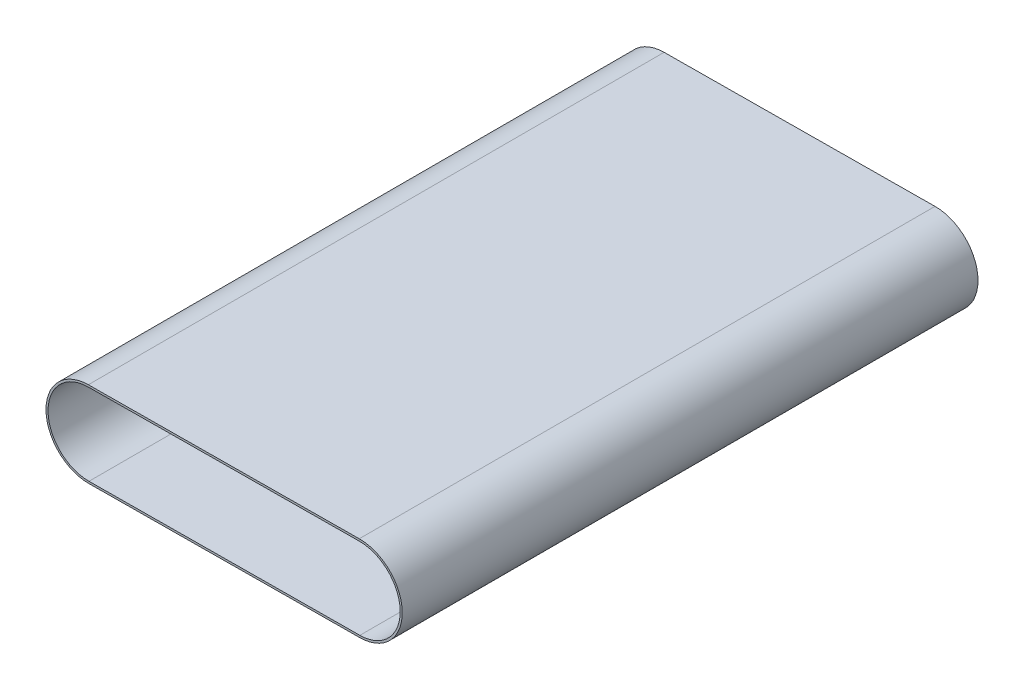
from build123d import *

# Parameters (mm, degrees)
EXTRUDE_1_DEPTH = 850


with BuildPart() as part:
    # 草图1 → 凸台-拉伸1 (new body)
    with BuildSketch(Plane.XY.offset(425)):
        with BuildLine():
            Line((662.463520786, 1437.017242521), (1062.402598848, 1440.036279946))
            ThreePointArc((1062.402598848, 1440.036279946), (1125.876361221, 1377.513632127), (1063.353713402, 1314.039869754))
            Line((1063.353713402, 1314.039869754), (663.414635339, 1311.020832329))
            ThreePointArc((663.414635339, 1311.020832329), (599.940872967, 1373.543480148), (662.463520786, 1437.017242521))
        make_face()
        with BuildLine():
            Line((662.48616637, 1434.017327992), (1062.425244433, 1437.036365417))
            ThreePointArc((1062.425244433, 1437.036365417), (1122.876446692, 1377.490986542), (1063.331067817, 1317.039784283))
            Line((1063.331067817, 1317.039784283), (663.391989755, 1314.020746858))
            ThreePointArc((663.391989755, 1314.020746858), (602.940787495, 1373.566125733), (662.48616637, 1434.017327992))
        make_face(mode=Mode.SUBTRACT)
    extrude(amount=-EXTRUDE_1_DEPTH)


solid = part.part
